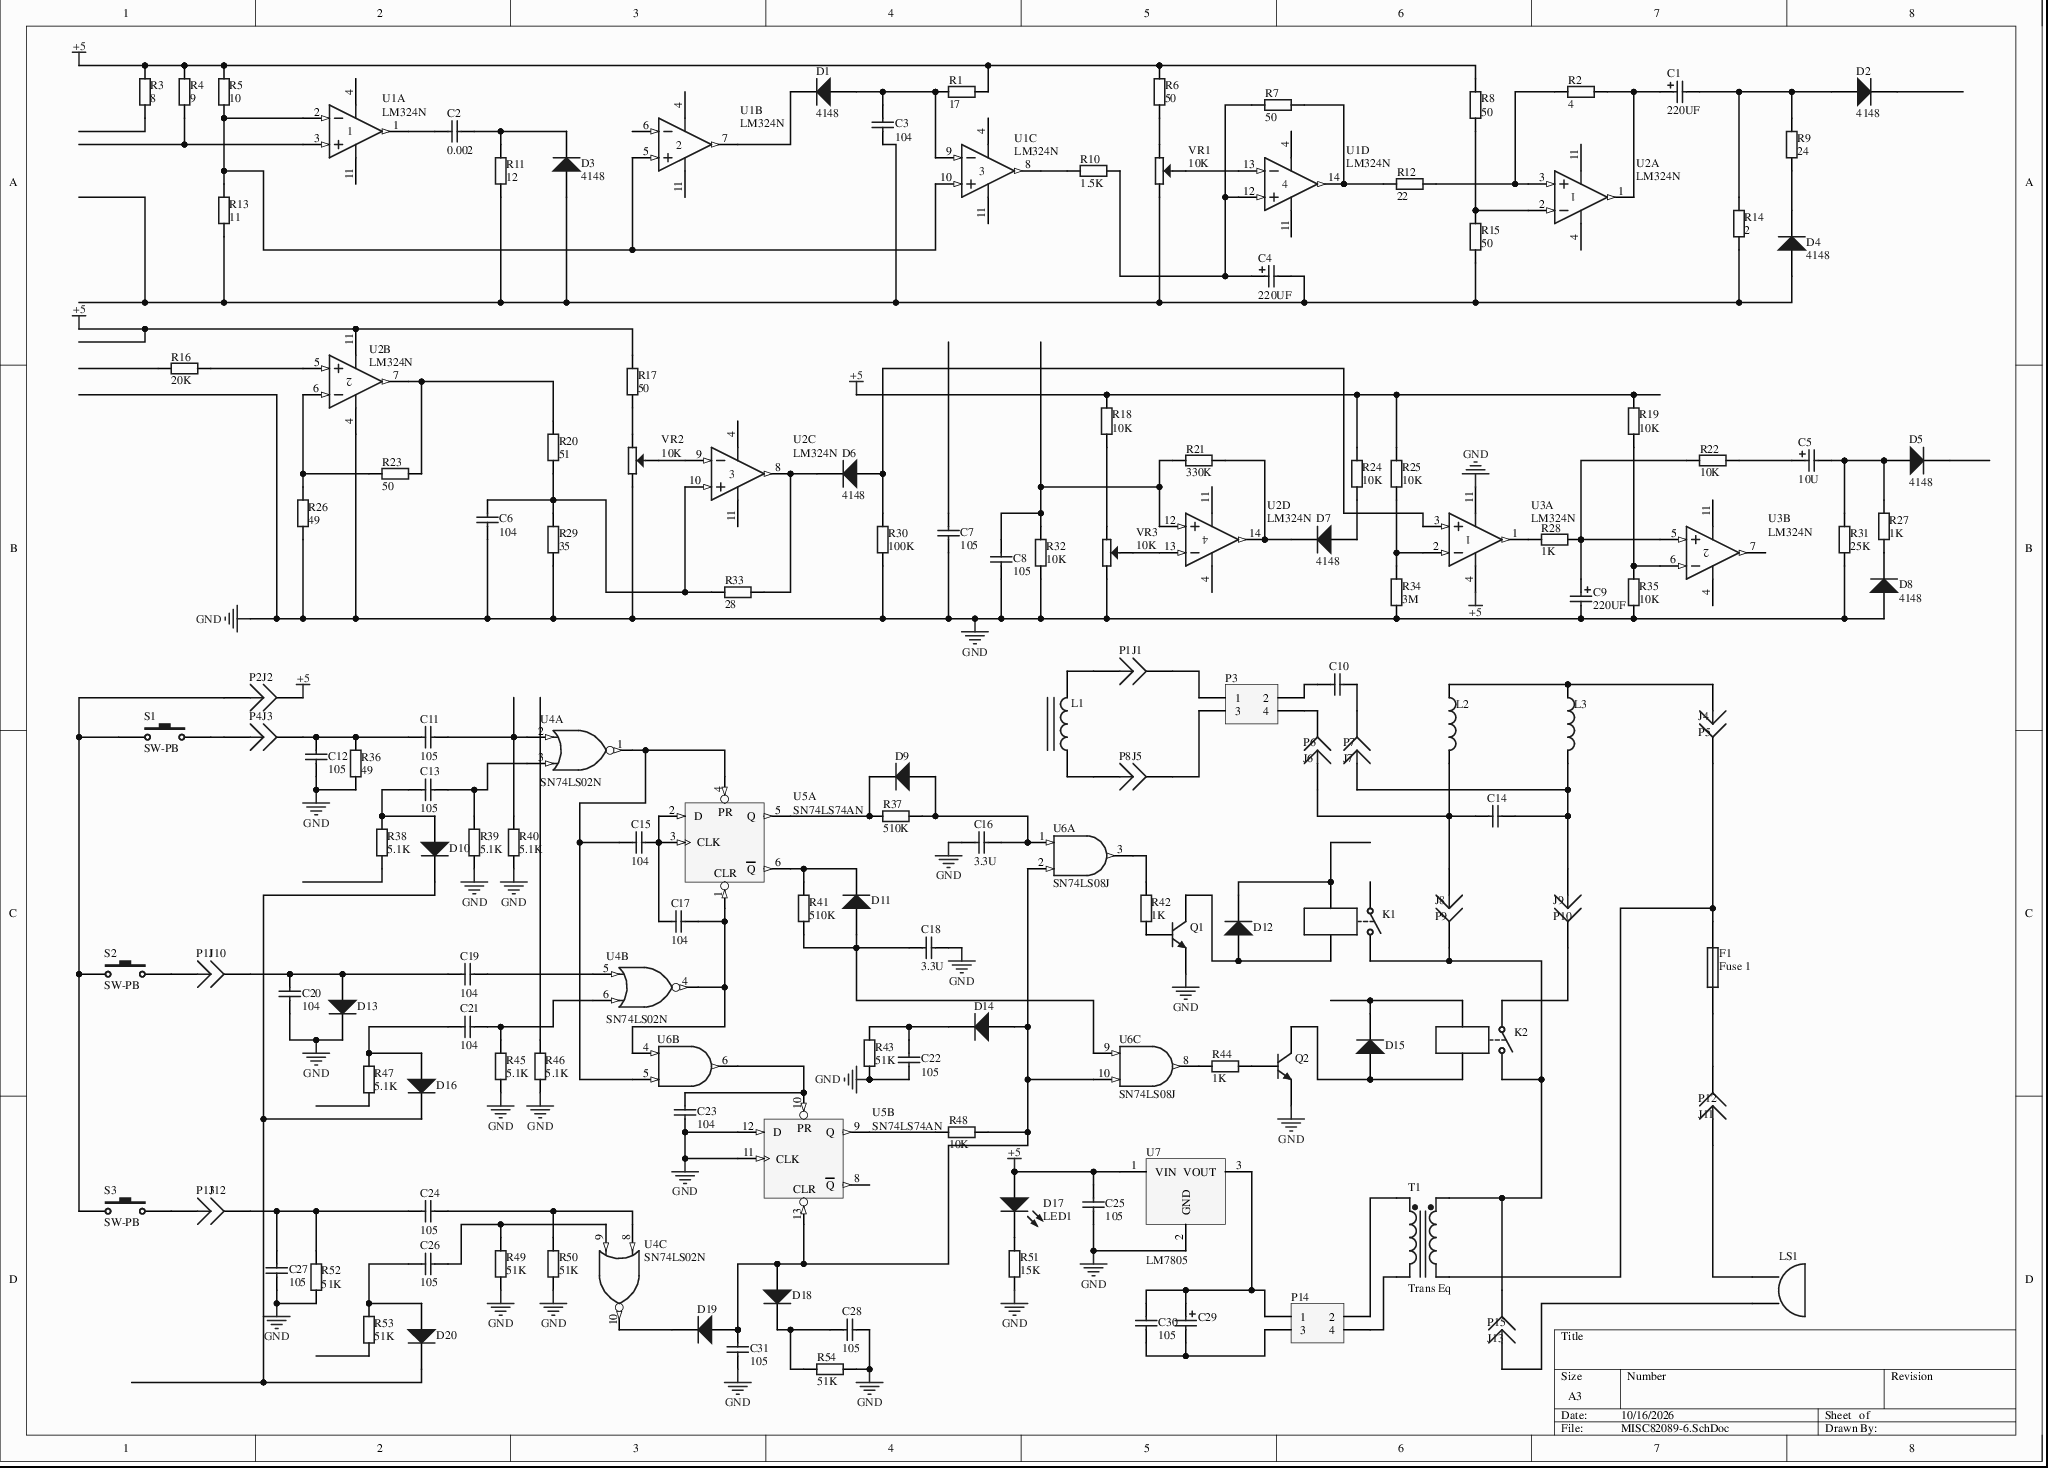
[diagram p0: MISC82089-6.SchDoc]
# Altium project MISC82089-2.PrjPcb
1 sheet, 156 parts. Net scope: global (net labels, ports and power ports of the same name join across sheets).
Board file: MISC82089.PcbDoc

## Sheet MISC82089-6.SchDoc
size A3

### Parts
C1  220UF  [POLAR0.8]
C2  0.002  [RAD-0.2]
C3  104  [RAD-0.2]
C4  220UF  [POLAR0.8]
C5  10U  [POLAR0.8]
C6  104  [RAD-0.2]
C7  105  [RAD-0.2]
C8  105  [RAD-0.2]
C9  220UF  [POLAR0.8]
C10  3.3U  [RAD-0.2]  (value not drawn)
C11  105  [RAD-0.2]
C12  105  [RAD-0.2]
C13  105  [RAD-0.2]
C14  3.3U  [RAD-0.2]  (value not drawn)
C15  104  [RAD-0.2]
C16  3.3U  [RAD-0.2]
C17  104  [RAD-0.2]
C18  3.3U  [RAD-0.2]
C19  104  [RAD-0.2]
C20  104  [RAD-0.2]
C21  104  [RAD-0.2]
C22  105  [RAD-0.2]
C23  104  [RAD-0.2]
C24  105  [RAD-0.2]
C25  105  [RAD-0.2]
C26  105  [RAD-0.2]
C27  105  [RAD-0.2]
C28  105  [RAD-0.2]
C29  220UF  [POLAR0.8]  (value not drawn)
C30  105  [RAD-0.2]
C31  105  [RAD-0.2]
D1  4148  [DO-35]
D2  4148  [DO-35]
D3  4148  [DO-35]
D4  4148  [DO-35]
D5  4148  [DO-35]
D6  4148  [DO-35]
D7  4148  [DO-35]
D8  4148  [DO-35]
D9  4148  [DO-35]  (value not drawn)
D10  4148  [DO-35]  (value not drawn)
D11  4148  [DO-35]  (value not drawn)
D12  4148  [DO-35]  (value not drawn)
D13  4148  [DO-35]  (value not drawn)
D14  4148  [DO-35]  (value not drawn)
D15  4148  [DO-35]  (value not drawn)
D16  4148  [DO-35]  (value not drawn)
D17  LED1  [LED-1]
D18  4148  [DO-35]  (value not drawn)
D19  4148  [DO-35]  (value not drawn)
D20  4148  [DO-35]  (value not drawn)
F1  Fuse 1  [PIN-W2/E2.8]
J1  Socket  [PIN1]  (value not drawn)
J2  Socket  [PIN1]  (value not drawn)
J3  Socket  [PIN1]  (value not drawn)
J4  Socket  [PIN1]  (value not drawn)
J5  Socket  [PIN1]  (value not drawn)
J6  Socket  [PIN1]  (value not drawn)
J7  Socket  [PIN1]  (value not drawn)
J8  Socket  [PIN1]  (value not drawn)
J9  Socket  [PIN1]  (value not drawn)
J10  Socket  [PIN1]  (value not drawn)
J11  Socket  [PIN1]  (value not drawn)
J12  Socket  [PIN1]  (value not drawn)
J13  Socket  [PIN1]  (value not drawn)
K1  Relay-SPST  [MODULE4]  (value not drawn)
K2  Relay-SPST  [MODULE4]  (value not drawn)
L1  Inductor Iron  [AXIAL-0.9]  (value not drawn)
L2  Inductor  [0402-A]  (value not drawn)
L3  Inductor  [0402-A]  (value not drawn)
LS1  Bell  [PIN2]  (value not drawn)
P1  Plug  [PIN1]  (value not drawn)
P2  Plug  [PIN1]  (value not drawn)
P3  Header 2X2  [HDR2X2]  (value not drawn)
P4  Plug  [PIN1]  (value not drawn)
P5  Plug  [PIN1]  (value not drawn)
P6  Plug  [PIN1]  (value not drawn)
P7  Plug  [PIN1]  (value not drawn)
P8  Plug  [PIN1]  (value not drawn)
P9  Plug  [PIN1]  (value not drawn)
P10  Plug  [PIN1]  (value not drawn)
P11  Plug  [PIN1]  (value not drawn)
P12  Plug  [PIN1]  (value not drawn)
P13  Plug  [PIN1]  (value not drawn)
P14  Header 2X2  [HDR2X2]  (value not drawn)
P15  Plug  [PIN1]  (value not drawn)
Q1  2N3904  [TO-92A]  (value not drawn)
Q2  2N3904  [TO-92A]  (value not drawn)
R1  17  [AXIAL-0.4]
R2  4  [AXIAL-0.4]
R3  8  [AXIAL-0.4]
R4  9  [AXIAL-0.4]
R5  10  [AXIAL-0.4]
R6  50  [AXIAL-0.4]
R7  50  [AXIAL-0.4]
R8  50  [AXIAL-0.4]
R9  24  [AXIAL-0.4]
R10  1.5K  [AXIAL-0.4]
R11  12  [AXIAL-0.4]
R12  22  [AXIAL-0.4]
R13  11  [AXIAL-0.4]
R14  2  [AXIAL-0.4]
R15  50  [AXIAL-0.4]
R16  20K  [AXIAL-0.4]
R17  50  [AXIAL-0.4]
R18  10K  [AXIAL-0.4]
R19  10K  [AXIAL-0.4]
R20  51  [AXIAL-0.4]
R21  330K  [AXIAL-0.4]
R22  10K  [AXIAL-0.4]
R23  50  [AXIAL-0.4]
R24  10K  [AXIAL-0.4]
R25  10K  [AXIAL-0.4]
R26  49  [AXIAL-0.4]
R27  1K  [AXIAL-0.4]
R28  1K  [AXIAL-0.4]
R29  35  [AXIAL-0.4]
R30  100K  [AXIAL-0.4]
R31  25K  [AXIAL-0.4]
R32  10K  [AXIAL-0.4]
R33  28  [AXIAL-0.4]
R34  3M  [AXIAL-0.4]
R35  10K  [AXIAL-0.4]
R36  49  [AXIAL-0.4]
R37  510K  [AXIAL-0.4]
R38  5.1K  [AXIAL-0.4]
R39  5.1K  [AXIAL-0.4]
R40  5.1K  [AXIAL-0.4]
R41  510K  [AXIAL-0.4]
R42  1K  [AXIAL-0.4]
R43  51K  [AXIAL-0.4]
R44  1K  [AXIAL-0.4]
R45  5.1K  [AXIAL-0.4]
R46  5.1K  [AXIAL-0.4]
R47  5.1K  [AXIAL-0.4]
R48  10K  [AXIAL-0.4]
R49  51K  [AXIAL-0.4]
R50  51K  [AXIAL-0.4]
R51  15K  [AXIAL-0.4]
R52  51K  [AXIAL-0.4]
R53  51K  [AXIAL-0.4]
R54  51K  [AXIAL-0.4]
S1  SW-PB  [SPST-2]
S2  SW-PB  [SPST-2]
S3  SW-PB  [SPST-2]
T1  Trans Eq  [TRF_4]
U1  LM324N  [646-06]  (parts A,B,C,D of 4)
U2  LM324N  [646-06]  (parts A,B,C,D of 4)
U3  LM324N  [646-06]  (parts A,B of 4)
U4  SN74LS02N  [N014]  (parts A,B,C of 4)
U5  SN74LS74AN  [646-06]  (parts A,B of 2)
U6  SN74LS08J  [J014]  (parts A,B,C of 4)
U7  LM7805  [TO220A]
VR1  10K  [3296W]
VR2  10K  [3296W]
VR3  10K  [3296W]

### Nets
+5: C25.2 D17.1(A) J2.1 R1.2 R3.2 R4.2 R5.2 R6.1 R8.2 R17.1 R18.1 R19.1 R24.1 R25.1 U2.11(V-) U3.4(V+) U7.1(VIN)
GND: C6.1 C7.2 C8.2 C9.2 C12.1 C16.1 C18.2 C20.1 C22.1 C23.1 C25.1 C27.2 C28.1 C31.2 D8.1(A) D13.2(K) Q1.1(E) Q2.1(E) R26.2 R29.2 R30.1 R31.2 R32.1 R34.2 R35.2 R36.2 R39.2 R40.2 R43.2 R45.2 R46.2 R49.2 R50.2 R51.1 R52.2 R54.2 U2.4(V+) U3.11(V-) U4.7(GND) U5.7(GND) U5.11(CLK) U5.12(D) U6.7(GND) U7.2(GND) VR2.2 VR3.2
VCC: U4.14(VCC) U6.14(VCC)
VDD: U5.14(VDD)
NetC1_1: C1.1 R2.1 U2.1(OUT)
NetC1_2: C1.2 D2.1(A) R9.1 R14.1
NetC2_1: C2.1 U1.1(OUT)
NetC2_2: C2.2 D3.2(K) R11.2
NetC3_1: C3.1 C4.2 D3.1(A) D4.1(A) R11.1 R13.1 R14.2 R15.1 VR1.2
NetC3_2: C3.2 D1.1(A) R1.1 U1.9(IN-)
NetC4_1: C4.1 R7.1 R10.2 U1.12(IN+)
NetC5_1: C5.1 R22.2
NetC5_2: C5.2 D5.1(A) R27.2 R31.1
NetC6_2: C6.2 R20.2 R29.1 R33.1 U2.10(IN+)
NetC8_1: C8.1 R21.1 R32.2 U2.12(IN+)
NetC9_1: C9.1 R22.1 R28.2 U3.5(IN+)
NetC10_1: C10.1 P3.2
NetC10_2: C10.2 J7.1
NetC11_1: C11.1 C12.2 J3.1 R36.1
NetC11_2: C11.2 R40.1 U4.2(A)
NetC13_1: C13.1 D10.1(A) R38.1
NetC13_2: C13.2 R39.1 U4.3(B)
NetC14_1: C14.1 L2.2 P6.1 P9.1
NetC14_2: C14.2 L3.2 P7.1 P10.1
NetC15_1: C15.1 U4.1(Y) U5.4(PR) U6.5(B)
NetC15_2: C15.2 C17.1 U5.2(D) U5.3(CLK)
NetC16_2: C16.2 D9.1(A) R37.2 U6.1(A)
NetC17_2: C17.2 U4.4(Y) U5.1(CLR) U6.4(A)
NetC18_1: C18.1 D11.1(A) R41.2 U6.9(A)
NetC19_1: C19.1 C20.2 D13.1(A) J10.1
NetC19_2: C19.2 U4.5(A)
NetC21_1: C21.1 D16.1(A) R47.1
NetC21_2: C21.2 R45.1 U4.6(B)
NetC22_2: C22.2 D14.2(K) R43.1
NetC23_2: C23.2 U5.10(PR) U6.6(Y)
NetC24_1: C24.1 R50.1 U4.8(A)
NetC24_2: C24.2 C27.1 J12.1 R52.1
NetC26_1: C26.1 R49.1 U4.9(B)
NetC26_2: C26.2 D20.1(A) R53.1
NetC28_2: C28.2 D18.2(K) R54.1
NetC29_1: C29.1 C30.2 P14.1 U7.3(VOUT)
NetC29_2: C29.2 C30.1 P14.3
NetC31_1: C31.1 D14.1(A) D18.1(A) D19.1(A) R48.2 U5.13(CLR) U6.2(B) U6.10(B)
NetD1_2: D1.2(K) U1.7(OUT)
NetD4_2: D4.2(K) R9.2
NetD6_1: D6.1(A) R30.2 U3.3(IN+)
NetD6_2: D6.2(K) R33.2 U2.8(OUT)
NetD7_1: D7.1(A) R24.2
NetD7_2: D7.2(K) R21.2 U2.14(OUT)
NetD8_2: D8.2(K) R27.1
NetD9_2: D9.2(K) R37.1 U5.5(Q)
NetD10_2: D10.2(K) D16.2(K) D20.2(K)
NetD11_2: D11.2(K) R41.1 U5.6(~{Q})
NetD12_1: D12.1(A) K1.4 Q1.3(C)
NetD12_2: D12.2(K) K1.3
NetD15_1: D15.1(A) K2.4 Q2.3(C)
NetD15_2: D15.2(K) K2.3
NetD17_2: D17.2(K) R51.2
NetD19_2: D19.2(K) U4.10(Y)
NetF1_1: F1.1 J11.1
NetF1_2: F1.2 J4.1 T1.4(Sec-)
NetJ1_1: J1.1 P3.1
NetJ5_1: J5.1 P3.3
NetJ6_1: J6.1 P3.4
NetJ8_1: J8.1 J13.1 K1.2 K2.2 T1.3(Sec+)
NetJ9_1: J9.1 K2.1
NetL1_1: L1.1 P8.1
NetL1_2: L1.2 P1.1
NetL2_1: L2.1 L3.1 P5.1
NetLS1_1: LS1.1(A) P12.1
NetLS1_2: LS1.2(B) P15.1
NetP2_1: P2.1 S1.1 S2.1 S3.1
NetP4_1: P4.1 S1.2
NetP11_1: P11.1 S2.2
NetP13_1: P13.1 S3.2
NetP14_2: P14.2 T1.1(Pri+)
NetP14_4: P14.4 T1.2(Pri-)
NetQ1_2: Q1.2(B) R42.2
NetQ2_2: Q2.2(B) R44.2
NetR2_2: R2.2 R12.2 U2.3(IN+)
NetR4_1: R4.1 U1.3(IN+)
NetR5_1: R5.1 R13.2 U1.2(IN-) U1.5(IN+) U1.10(IN+)
NetR6_2: R6.2 VR1.1
NetR7_2: R7.2 R12.1 U1.14(OUT)
NetR8_1: R8.1 R15.2 U2.2(IN-)
NetR10_1: R10.1 U1.8(OUT)
NetR16_1: R16.1 U2.5(IN+)
NetR17_2: R17.2 VR2.1
NetR18_2: R18.2 VR3.1
NetR19_2: R19.2 R35.1 U3.6(IN-)
NetR20_1: R20.1 R23.1 U2.7(OUT)
NetR23_2: R23.2 R26.1 U2.6(IN-)
NetR25_2: R25.2 R34.1 U3.2(IN-)
NetR28_1: R28.1 U3.1(OUT)
NetR42_1: R42.1 U6.3(Y)
NetR44_1: R44.1 U6.8(Y)
NetR48_1: R48.1 U5.9(Q)
NetU1_13: U1.13(IN-) VR1.2
NetU2_9: U2.9(IN-) VR2.2
NetU2_13: U2.13(IN-) VR3.2

Not connected (* = marked no-connect by the designer): C7 1; D2 2(K); D5 2(K); K1 1; R3 1; R16 2; R38 2; R46 1; R47 2; R53 2; U1 4(V+) 6(IN-) 11(V-); U3 7(OUT); U5 8(~{Q})

### Library data of the parts
C1 C4 C5 C9 C29 = Cap Pol2: Polarized Capacitor (Axial); Value: 100pF; Published: 8-Jun-2000; LatestRevisionDate: 17-Jul-2002; LatestRevisionNote: Re-released for DXP Platform.; PackageReference: POLAR0.8; PackageDescription: Polarized Capacitor; 2 Leads; Publisher: Altium Limited
C2 C3 C6-C8 C10-C28 C30 C31 = Cap: Capacitor; Value: 100pF; Published: 8-Jun-2000; LatestRevisionDate: 17-Jul-2002; LatestRevisionNote: Re-released for DXP Platform.; PackageReference: RAD-0.3; PackageDescription: Radial Cap, Thru-Hole; 2 Leads; 0.3 in Pin Spacing; Publisher: Altium Limited
D1-D16 D18-D20 = Diode 1N914: High Conductance Fast Diode; Published: 8-Jun-2000; LatestRevisionDate: 17-Jul-2002; LatestRevisionNote: Re-released for DXP Platform.; DatasheetVersion: 1997; PackageReference: DO-35; PackageDescription: Diode, Axial; Body 3.8 x 1.9 mm (LxDia. max), Lead Dia. 0.53 mm (max); Code_JEDEC: DO-204-AH; ComponentLink1Description: Manufacturer Link; ComponentLink2Description: Datasheet; ComponentLink2URL: http://www.fairchildsemi.com/ds/1N%2F1N4448.pdf; Publisher: Altium Limited
D17 = LED1: Typical RED GaAs LED; Published: 8-Jun-2000; LatestRevisionDate: 08-Jul-2005; LatestRevisionNote: Mech Layer 1 removed.; PackageReference: LED-1; PackageDescription: LED; 2 Leads; Publisher: Altium Limited
F1 = Fuse 1: Fuse; Published: 8-Jun-2000; LatestRevisionDate: 17-Jul-2002; LatestRevisionNote: Re-released for DXP Platform.; PackageReference: PIN-W2/E2.8; PackageDescription: Thru-Hole; 2 Leads; Publisher: Altium Limited
K1 K2 = Relay-SPST: Single-Pole Single-Throw Relay; Published: 24-Mar-1999; LatestRevisionDate: 17-Jul-2002; LatestRevisionNote: Re-released for DXP Platform.; PackageReference: MODULE4; Publisher: Altium Limited
L1 = Inductor Iron: Magnetic-Core Inductor; Value: 10mH; Published: 24-Mar-1999; LatestRevisionDate: 17-Jul-2002; LatestRevisionNote: Re-released for DXP Platform.; PackageReference: AXIAL-0.9; PackageDescription: Axial Device, Thru-Hole; 2 Leads; 0.9 in Pin Spacing; Publisher: Altium Limited
L2 L3 = Inductor: Code_IEC: 1005; Value: 10mH; Published: 8-Jun-2000; LatestRevisionDate: 29-May-2009; LatestRevisionNote: IPC-7351 Footprint Added.; PackageReference: 0402-A; PackageDescription: Chip Inductor; Code_JEITA: 0402; Publisher: Altium Limited
LS1 = Bell: Electrical Bell; Published: 24-Mar-1999; LatestRevisionDate: 17-Jul-2002; LatestRevisionNote: Re-released for DXP Platform.; PackageReference: PIN2; Publisher: Altium Limited
P3 P14 = Header 2X2: Header, 2-Pin, Dual row; LatestRevisionDate: 17-Jul-2002; LatestRevisionNote: Re-released for DXP Platform.; Publisher: Altium Limited
Q1 Q2 = 2N3904: NPN General Purpose Amplifier; Published: 8-Jun-2000; LatestRevisionDate: 15-Jan-2003; LatestRevisionNote: PCB Footprint 'BCY-W3/D4.7' replaced; DatasheetVersion: 1997; PackageVersion: Sep-1998; PackageReference: TO-92A; PackageDescription: TO, Flat Index; 3 In-Line, Axial Leads; Body Dia. 4.5mm; Leads 0.51 x 0.48 mm (max); ComponentLink1Description: Manufacturer Link; ComponentLink2Description: Datasheet; ComponentLink2URL: http://www.fairchildsemi.com/ds/2N%2F2N3904.pdf; Publisher: Altium Limited
R1-R26 R29-R41 R43 R45-R54 = Res2: Resistor; Value: 1K; Published: 8-Jun-2000; LatestRevisionDate: 17-Jul-2002; LatestRevisionNote: Re-released for DXP Platform.; PackageReference: AXIAL-0.4; PackageDescription: Axial Device, Thru-Hole; 2 Leads; 0.4 in Pin Spacing; Publisher: Altium Limited
R27 R28 R42 R44 = Res2: Resistor; Published: 8-Jun-2000; LatestRevisionDate: 17-Jul-2002; LatestRevisionNote: Re-released for DXP Platform.; PackageReference: AXIAL-0.4; PackageDescription: Axial Device, Thru-Hole; 2 Leads; 0.4 in Pin Spacing; Value: 1K; Publisher: Altium Limited
S1-S3 = SW-PB: Switch; Published: 24-Mar-1999; LatestRevisionDate: 17-Jul-2002; LatestRevisionNote: Re-released for DXP Platform.; PackageReference: SPST-2; PackageDescription: Switch; 2 Leads; Publisher: Altium Limited
T1 = Trans Eq: Transformer (Equivalent Circuit Model); Published: 8-Jun-2000; LatestRevisionDate: 17-Jul-2002; LatestRevisionNote: Re-released for DXP Platform.; PackageReference: TRF_4; PackageDescription: Transformer; 4 Leads; Publisher: Altium Limited
U1-U3 = LM324N: Quad Low-Power Operational Amplifier; Package Information: Latest Revision: 1997; Published: 17-Jul-2002; Datasheet: Linear and Interface Integrated Circuits, DL128 Rev2 (1988); Package Reference: 646-06; Publisher: Altium Limited
U4 = SN74LS02N: Quadruple 2-Input Positive-NOR Gate; Package Information: Latest Revision: Oct-1995; Published: 8-Jun-2000; Revision: 17-Jul-2002: Re-released for DXP Platform.; Datasheet: Latest Revision: Mar-1988; Package Reference: N014; Publisher: Altium Limited
U5 = SN74LS74AN: Dual D-Type Positive Edge-Triggered Flip-Flop; Package Information: Latest Revision: 1995; Published: 15-Apr-2002; Datasheet: Latest Revision: Dec-1999; Package Reference: 646-06; Publisher: Altium Limited
U6 = SN74LS08J: Quadruple 2-Input Positive-AND Gate; Package Information: Latest Revision: Jun-1999; Published: 8-Jun-2000; Revision: 17-Jul-2002: Re-released for DXP Platform.; Datasheet: Latest Revision: Mar-1988; Package Reference: J014; Publisher: Altium Limited
VR1-VR3 = RESVR
J1-J13 = Socket: LatestRevisionDate: 17-Jul-2002; LatestRevisionNote: Re-released for DXP Platform.; Publisher: Altium Limited
P1 P2 P4-P13 P15 = Plug: LatestRevisionDate: 17-Jul-2002; LatestRevisionNote: Re-released for DXP Platform.; Publisher: Altium Limited